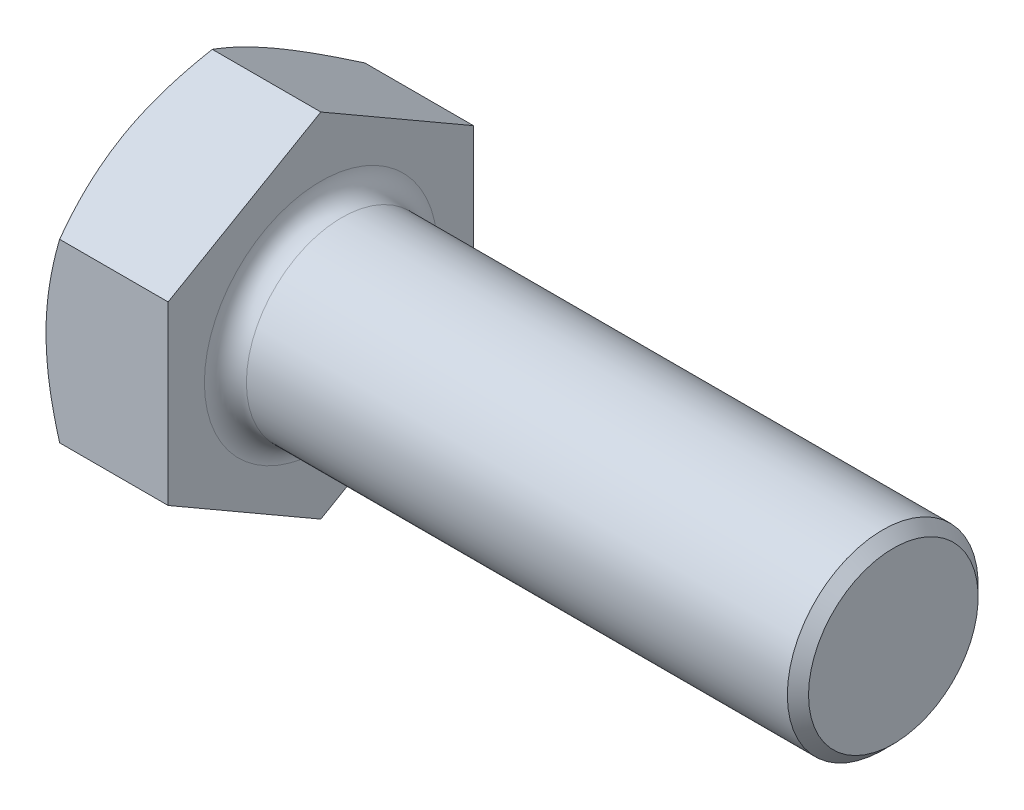
from build123d import *

# Parameters (mm, degrees)
BOSS_EXTRUDE1_DEPTH = 6.4
SKETCH4_R           = 17.59
SKETCH4_R_2         = 8
CUT_EXTRUDE1_DEPTH  = 0.8
CUT_EXTRUDE1_DRAFT  = -60
CHAMFER2_SIZE       = 0.555555556


with BuildPart() as part:
    # Sketch3 → Boss-Extrude1 (new body)
    with BuildSketch(Plane(origin=(0, 0, 0), x_dir=(0, 0, -1), z_dir=(1, 0, 0))):
        Polygon((8, 4.618802154), (0, 9.237604307), (-8, 4.618802154), (-8, -4.618802154), (0, -9.237604307), (8, -4.618802154), align=None)
    extrude(amount=BOSS_EXTRUDE1_DEPTH)


with BuildPart() as cut_extrude1_tool:
    # Sketch4 → Cut-Extrude1 (with draft: the straight prism first)
    with BuildSketch(Plane.ZY):
        Circle(SKETCH4_R)
        Circle(SKETCH4_R_2, mode=Mode.SUBTRACT)
    extrude(amount=-CUT_EXTRUDE1_DEPTH)
    # Cut-Extrude1: the draft: its side faces are tilted about the plane it starts from
    cut_extrude1_sides = [cut_extrude1_tool.faces().sort_by_distance(p)[0] for p in [
        (0.4, 0, -17.59),
        (0.4, 0, -8),
    ]]
    draft(cut_extrude1_sides, Plane.ZY, CUT_EXTRUDE1_DRAFT)


with BuildPart() as part_1:
    add(part.part)

    # Cut-Extrude1: cut by cut_extrude1_tool
    add(cut_extrude1_tool.part, mode=Mode.SUBTRACT)

    # Sketch5 → Revolve1 (revolve)
    with BuildSketch(Plane.XY, mode=Mode.PRIVATE) as revolve1_sk:
        with BuildLine():
            Line((7.5, 5), (36.4, 5))
            Line((36.4, 5), (36.4, 0))
            Line((36.4, 0), (6.4, 0))
            Line((6.4, 0), (6.4, 6.1))
            ThreePointArc((6.4, 6.1), (6.722182541, 5.322182541), (7.5, 5))
        make_face()
    revolve(revolve1_sk.sketch.rotate(Axis((6.4, 0, 0), (1, 0, 0)), 90), axis=Axis((6.4, 0, 0), (1, 0, 0)))

    # Chamfer2
    chamfer2_edges = [part_1.edges().sort_by_distance(p)[0] for p in [
        (36.4, 0, -5),
    ]]
    chamfer(chamfer2_edges, length=CHAMFER2_SIZE)


solid = part_1.part
